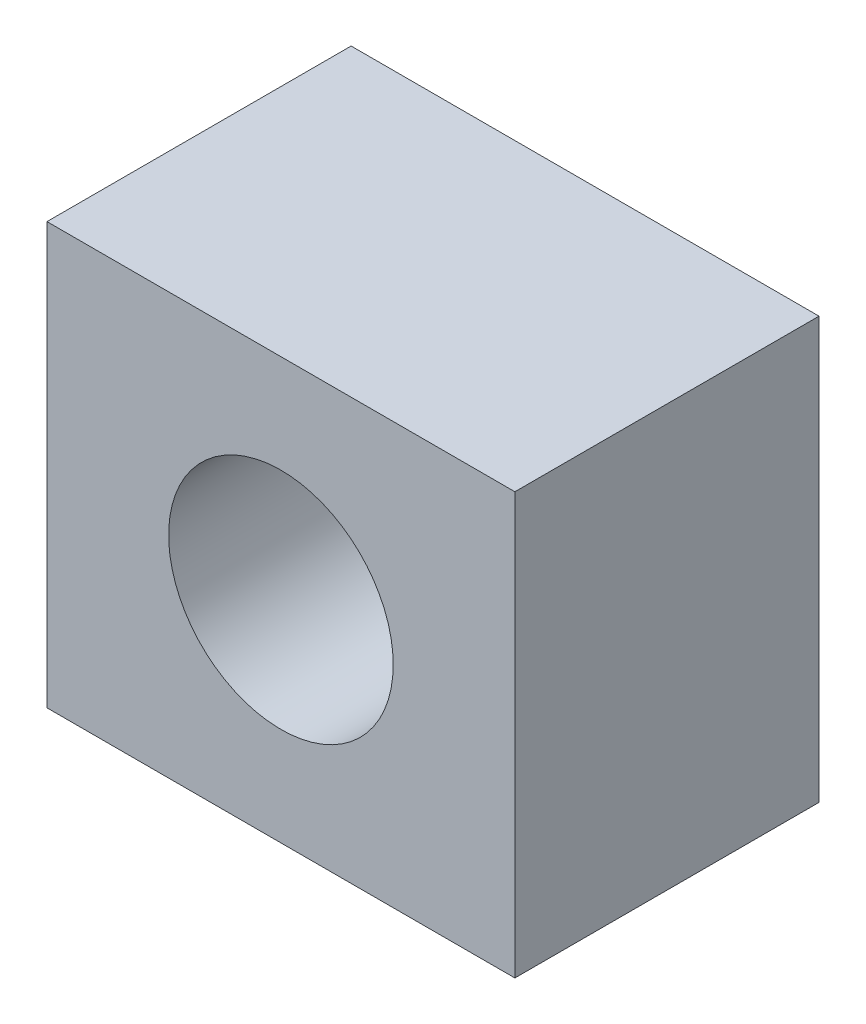
SolidWorks part; units mm, degrees
material "45"
ref_plane "Front Plane" through (0, 0, 0) normal (0, 0, 1) x (1, 0, 0)
ref_plane "Top Plane" through (0, 0, 0) normal (0, 1, 0) x (1, 0, 0)
ref_plane "Right Plane" through (0, 0, 0) normal (1, 0, 0) x (0, 0, -1)
sketch "Sketch1" plane through (0, 0, 0) normal (0, 0, 1) x (1, 0, 0)
  line L1 (0, 0) -> (100, 0)
  line L2 (0, 0) -> (0, 90)
  line L3 (0, 90) -> (100, 90)
  line L4 (100, 0) -> (100, 90)
  circle A0 centre (50, 45) radius 24
  dimension "D3" = 48
  dimension "D4" = 45
  dimension "D5" = 50
  dimension "D1" = 100
  dimension "D2" = 90
extrude "Boss-Extrude1" add sketch "Sketch1" along normal blind 65
cosmetic thread "Cosmetic Thread1" parameters "D2"=68
